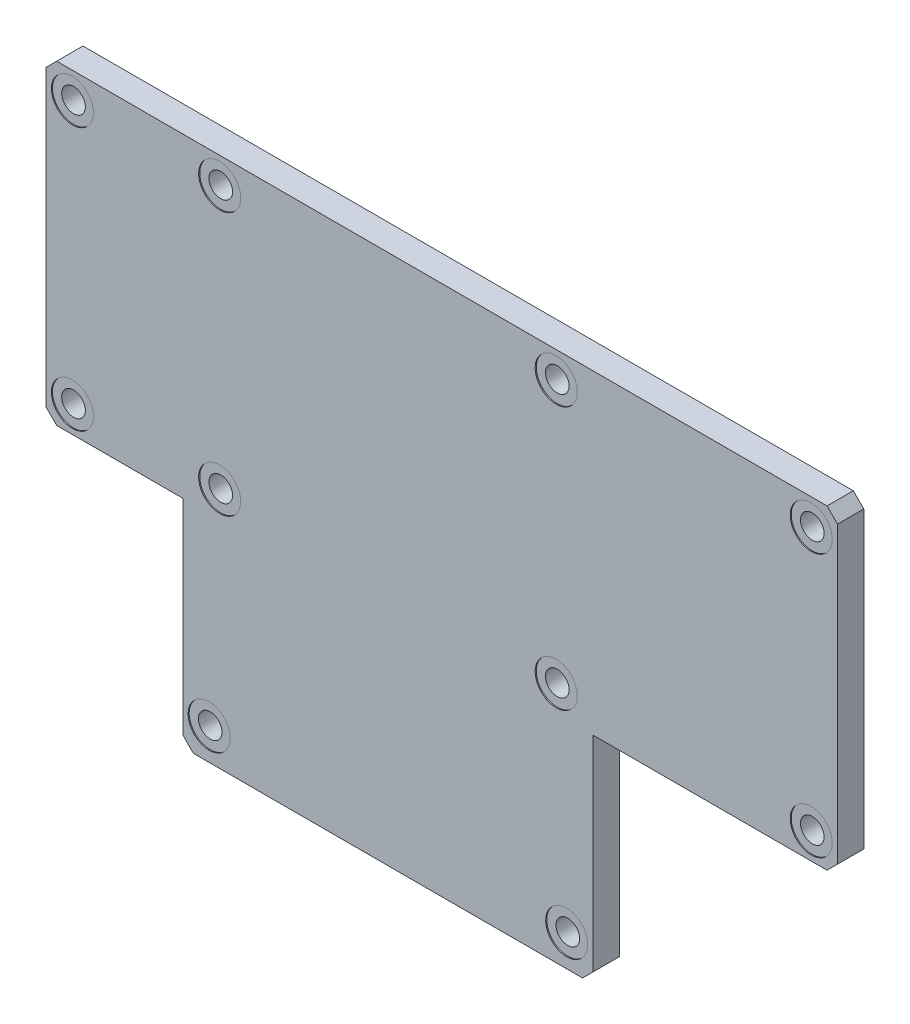
from build123d import *

# Parameters (mm, degrees)
BOSS_EXTRUDE1_DEPTH = 50
HOLE1_D             = 45
HOLE1_CBORE_D       = 80
HOLE1_CBORE_DEPTH   = 2
CHAMFER1_SIZE       = 20


with BuildPart() as part:
    # Sketch1 → Boss-Extrude1 (new body)
    with BuildSketch(Plane.XY):
        Polygon((390, 410), (855, 410), (855, 1010), (-650, 1010), (-650, 410), (-390, 410), (-390, 0), (390, 0), align=None)
    extrude(amount=BOSS_EXTRUDE1_DEPTH)

    # Hole1 (through all)
    with Locations(Plane.XY.offset(50)):
        with Locations((-600, 960), (320, 960), (805, 960), (-340, 60), (340, 60), (-320, 960), (805, 460), (320, 460), (-320, 460), (-600, 460)):
            CounterBoreHole(HOLE1_D / 2, HOLE1_CBORE_D / 2, HOLE1_CBORE_DEPTH)

    # Chamfer1
    chamfer1_edges = [part.edges().sort_by_distance(p)[0] for p in [
        (-650, 410, 25),
        (-650, 1010, 25),
        (855, 1010, 25),
        (855, 410, 25),
        (390, 0, 25),
        (-390, 0, 25),
    ]]
    chamfer(chamfer1_edges, length=CHAMFER1_SIZE)


solid = part.part
